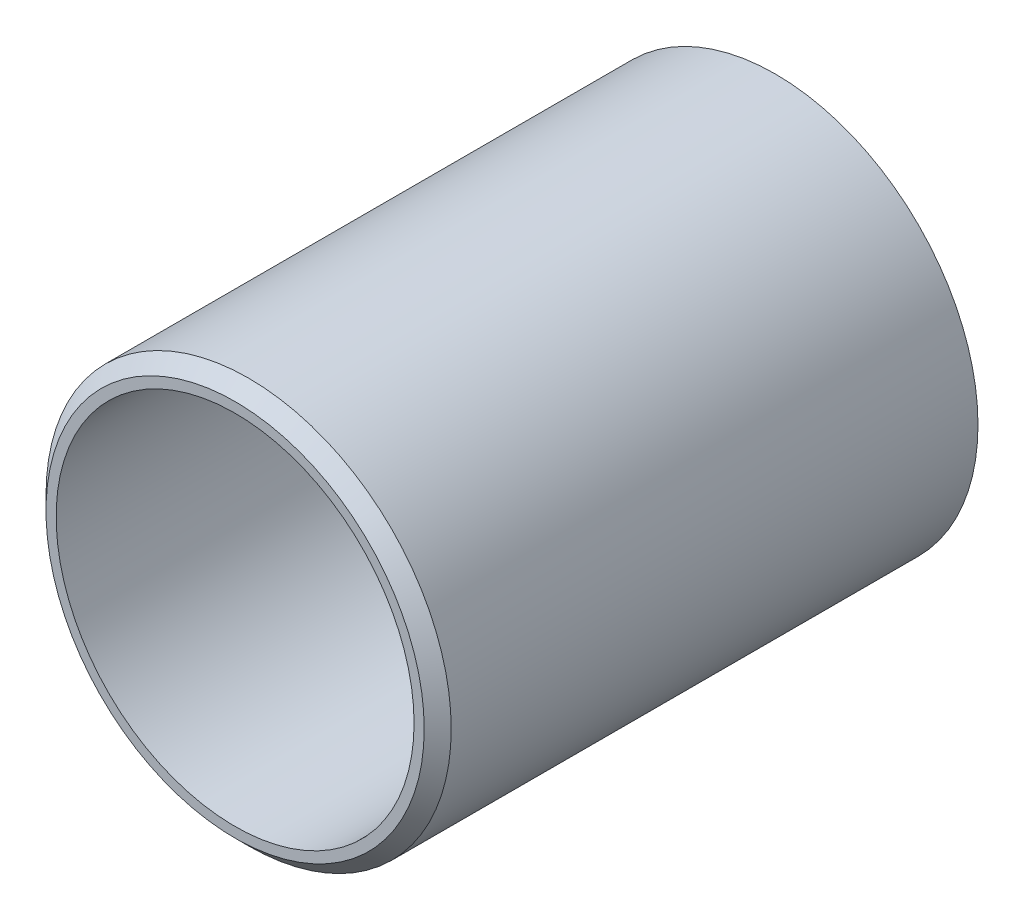
from build123d import *

# Parameters (mm, degrees)
SKETCH_1_R      = 30
SKETCH_1_R_2    = 26.5
EXTRUDE_1_DEPTH = 80
CHAMFER_1_SIZE  = 2


with BuildPart() as part:
    # 草图1 → 拉伸1 (new body)
    with BuildSketch(Plane.XY):
        Circle(SKETCH_1_R)
        Circle(SKETCH_1_R_2, mode=Mode.SUBTRACT)
    extrude(amount=EXTRUDE_1_DEPTH)

    # 倒角1
    chamfer_1_edges = [part.edges().sort_by_distance(p)[0] for p in [
        (-30, 0, 80),
    ]]
    chamfer(chamfer_1_edges, length=CHAMFER_1_SIZE)


solid = part.part
